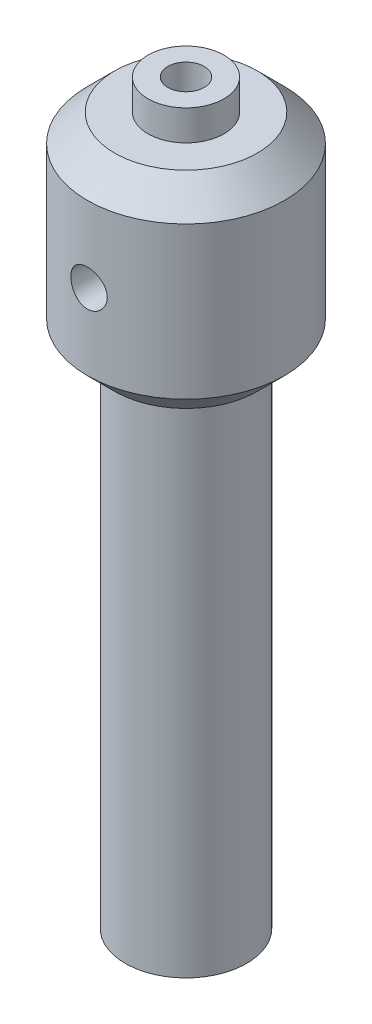
from build123d import *

# Parameters (mm, degrees)
SKETCH1_W          = 20
SKETCH1_H          = 165
SKETCH1_W_2        = 32.5
SKETCH1_H_2        = 50
SKETCH1_W_3        = 12.5
SKETCH1_H_3        = 10
SKETCH6_R          = 6
CUT_EXTRUDE1_DEPTH = 80


with BuildPart() as part:
    # Sketch1 → Revolve7 (revolve)
    with BuildSketch(Plane.XY, mode=Mode.PRIVATE) as revolve7_sk:
        with Locations((10, -108.875)):
            Rectangle(SKETCH1_W, SKETCH1_H)
        Polygon((0, -26.375), (23.5, -26.375), (32.5, -17.375), (0, -17.375), align=None)
        with Locations((16.25, 7.625)):
            Rectangle(SKETCH1_W_2, SKETCH1_H_2)
        Polygon((0, 32.625), (0, 41.625), (23.5, 41.625), (32.5, 32.625), align=None)
        with Locations((6.25, 46.625)):
            Rectangle(SKETCH1_W_3, SKETCH1_H_3)
    revolve(revolve7_sk.sketch.rotate(Axis((0, -26.375, 0), (0, -1, 0)), 180), axis=Axis((0, -26.375, 0), (0, -1, 0)))

    # Sketch5 → Cut-Revolve1 (revolve, cut)
    with BuildSketch(Plane.XY, mode=Mode.PRIVATE) as cut_revolve1_sk:
        Polygon((0, 51.625), (0, 24.625), (0, 21.625), (6, 24.625), (6, 51.625), align=None)
    revolve(cut_revolve1_sk.sketch.rotate(Axis((0, 51.625, 0), (0, -1, 0)), 180), axis=Axis((0, 51.625, 0), (0, -1, 0)), mode=Mode.SUBTRACT)

    # Sketch6 → Cut-Extrude1 (cut, symmetric)
    with BuildSketch(Plane.XY):
        with Locations((0, 7.625)):
            Circle(SKETCH6_R)
    extrude(amount=CUT_EXTRUDE1_DEPTH, both=True, mode=Mode.SUBTRACT)


solid = part.part
